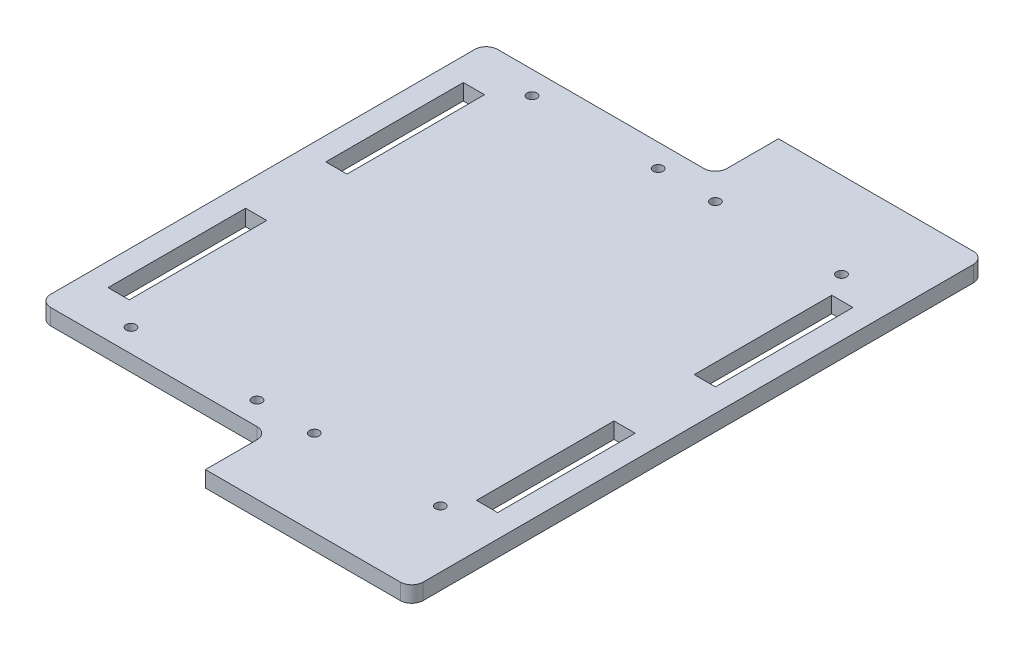
from build123d import *

# Parameters (mm, degrees)
SKETCH1_W                   = 380
SKETCH1_H                   = 500
BOSS_EXTRUDE1_DEPTH         = 14
SKETCH2_W                   = 200
SKETCH2_H                   = 55
CUT_EXTRUDE1_DEPTH          = 14
FILLET1_R                   = 10
SKETCH3_W                   = 18.5
SKETCH3_H                   = 120
CUT_EXTRUDE2_DEPTH          = 20
M10_TAPPED_HOLE1_AT_2_COUNT = 2
M10_TAPPED_HOLE1_AT_2_PITCH = 110
M10_TAPPED_HOLE1_AT_3_COUNT = 2
M10_TAPPED_HOLE1_AT_3_PITCH = 366.878726557
M10_TAPPED_HOLE1_AT_4_COUNT = 2
M10_TAPPED_HOLE1_AT_4_PITCH = 350
LPATTERN1_COUNT             = 2
LPATTERN1_PITCH             = 160
FILLET2_R                   = 10


with BuildPart() as part:
    # Sketch1 → Boss-Extrude1 (new body)
    with BuildSketch(Plane(origin=(0, 0, 0), x_dir=(1, 0, 0), z_dir=(0, 1, 0))):
        Rectangle(SKETCH1_W, SKETCH1_H)
    extrude(amount=BOSS_EXTRUDE1_DEPTH)

    # Sketch2 → Cut-Extrude1 (cut)
    with BuildSketch(Plane(origin=(0, 14, 0), x_dir=(1, 0, 0), z_dir=(0, 1, 0))):
        with Locations((-90, 222.5)):
            Rectangle(SKETCH2_W, SKETCH2_H)
        with Locations((-90, -222.5)):
            Rectangle(SKETCH2_W, SKETCH2_H)
    extrude(amount=-CUT_EXTRUDE1_DEPTH, mode=Mode.SUBTRACT)

    # Fillet1
    fillet1_edges = [part.edges().sort_by_distance(p)[0] for p in [
        (10, 7, -195),
        (10, 7, 195),
    ]]
    fillet(fillet1_edges, radius=FILLET1_R)

    # Sketch3 → Cut-Extrude2 (cut)
    with BuildSketch(Plane(origin=(0, 14, 0), x_dir=(1, 0, 0), z_dir=(0, 1, 0))):
        with Locations((160.75, 95)):
            Rectangle(SKETCH3_W, SKETCH3_H)
        with Locations((160.75, -95)):
            Rectangle(SKETCH3_W, SKETCH3_H)
        with Locations((-160.75, -95)):
            Rectangle(SKETCH3_W, SKETCH3_H)
        with Locations((-160.75, 95)):
            Rectangle(SKETCH3_W, SKETCH3_H)
    extrude(amount=-CUT_EXTRUDE2_DEPTH, mode=Mode.SUBTRACT)

    # Sketch5 → M10 Tapped Hole1 (revolve, cut)
    with BuildSketch(Plane(origin=(30, 14, 175), x_dir=(0, 0, 1), z_dir=(1, 0, 0))):
        Polygon((0, 0), (0, 55.553657631), (4.25, 53), (4.25, 0), align=None)
    m10_tapped_hole1 = revolve(axis=Axis((30, 20.35, 175), (0, -1, 0)), mode=Mode.SUBTRACT)

    # M10 Tapped Hole1 at 2: M10 Tapped Hole1 ×2
    with Locations(*[(i * M10_TAPPED_HOLE1_AT_2_PITCH, 0, 0) for i in range(1, M10_TAPPED_HOLE1_AT_2_COUNT)]):
        add(m10_tapped_hole1, mode=Mode.SUBTRACT)

    # M10 Tapped Hole1 at 3: M10 Tapped Hole1 ×2
    with Locations(*[Vector(0.29982659674039447, 0, -0.9539937169012556) * (i * M10_TAPPED_HOLE1_AT_3_PITCH) for i in range(1, M10_TAPPED_HOLE1_AT_3_COUNT)]):
        add(m10_tapped_hole1, mode=Mode.SUBTRACT)

    # M10 Tapped Hole1 at 4: M10 Tapped Hole1 ×2
    with Locations(*[(0, 0, -i * M10_TAPPED_HOLE1_AT_4_PITCH) for i in range(1, M10_TAPPED_HOLE1_AT_4_COUNT)]):
        add(m10_tapped_hole1, mode=Mode.SUBTRACT)

    # LPattern1: M10 Tapped Hole1 ×2
    with Locations(*[(-i * LPATTERN1_PITCH, 0, 0) for i in range(1, LPATTERN1_COUNT)]):
        add(m10_tapped_hole1, mode=Mode.SUBTRACT)

    # LPattern1 copy 1 sketch → LPattern1 copy 1 (revolve, cut)
    with BuildSketch(Plane(origin=(-20, 14, 175), x_dir=(0, 0, 1), z_dir=(1, 0, 0))):
        Polygon((0, 0), (0, 55.553657631), (4.25, 53), (4.25, 0), align=None)
    revolve(axis=Axis((-20, 20.35, 175), (0, -1, 0)), mode=Mode.SUBTRACT)

    # LPattern1 copy 2 sketch → LPattern1 copy 2 (revolve, cut)
    with BuildSketch(Plane(origin=(-20, 14, -175), x_dir=(0, 0, 1), z_dir=(1, 0, 0))):
        Polygon((0, 0), (0, 55.553657631), (4.25, 53), (4.25, 0), align=None)
    revolve(axis=Axis((-20, 20.35, -175), (0, -1, 0)), mode=Mode.SUBTRACT)

    # LPattern1 copy 3 sketch → LPattern1 copy 3 (revolve, cut)
    with BuildSketch(Plane(origin=(-130, 14, -175), x_dir=(0, 0, 1), z_dir=(1, 0, 0))):
        Polygon((0, 0), (0, 55.553657631), (4.25, 53), (4.25, 0), align=None)
    revolve(axis=Axis((-130, 20.35, -175), (0, -1, 0)), mode=Mode.SUBTRACT)

    # Fillet2
    fillet2_edges = [part.edges().sort_by_distance(p)[0] for p in [
        (-190, 7, -195),
        (-190, 7, 195),
        (190, 7, 250),
        (190, 7, -250),
    ]]
    fillet(fillet2_edges, radius=FILLET2_R)


solid = part.part
